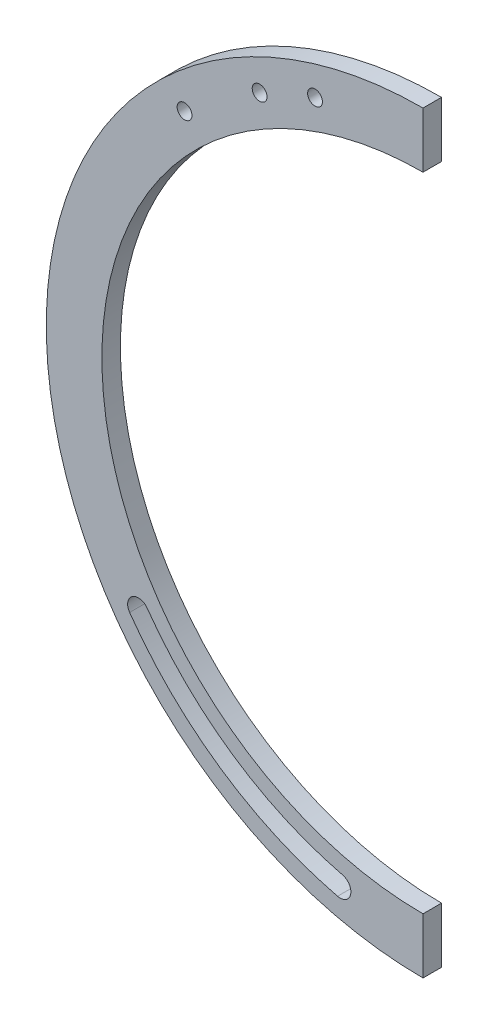
SolidWorks part; units mm, degrees
ref_plane "Front Plane" through (0, 0, 0) normal (0, 0, 1) x (1, 0, 0)
ref_plane "Top Plane" through (0, 0, 0) normal (0, 1, 0) x (1, 0, 0)
ref_plane "Right Plane" through (0, 0, 0) normal (1, 0, 0) x (0, 0, -1)
sketch "Sketch1" plane through (0, 0, 0) normal (0, 0, 1) x (1, 0, 0)
  circle A0 centre (291.5852, 182.7307) radius 203.2949
  circle A1 centre (291.5852, 182.7307) radius 173.2949
  arc A2 (93.8621, 230) -> (110.6713, 90) centre (291.5852, 182.7307) ccw construction
  dimension "D1" = 30
extrude "Boss-Extrude1" add sketch "Sketch1" against normal blind 10
sketch "Sketch2" plane through (0, 0, -10) normal (0, 0, -1) x (-1, 0, 0)
  line L0 (-291.5852, 9.4358) -> (-291.5852, -33.9055)
  line L1 (-291.5852, 356.0256) -> (-291.5852, 399.3669)
  circle A0 centre (-291.5852, 182.7307) radius 173.2949 construction
  arc A1 (-291.5852, 356.0256) -> (-291.5852, 9.4358) centre (-291.5852, 182.7307) ccw
  arc A2 (-291.5852, 399.3669) -> (-291.5852, -33.9055) centre (-291.5852, 182.7307) ccw
extrude "Cut-Extrude1" cut sketch "Sketch2" against normal blind 185
sketch "Sketch3" plane through (0, 0, -10) normal (0, 0, -1) x (-1, 0, 0)
  arc A0 (-246.849, 0.2333) -> (-138.0051, 74.4728) centre (-291.5852, 182.7307) ccw construction
  arc A1 (-245.4633, -5.4196) -> (-133.2479, 71.1194) centre (-291.5852, 182.7307) ccw
  arc A2 (-248.2347, 5.8862) -> (-142.7622, 77.8261) centre (-291.5852, 182.7307) ccw
  arc A3 (-248.2347, 5.8862) -> (-245.4633, -5.4196) centre (-246.849, 0.2333) ccw
  arc A4 (-133.2479, 71.1194) -> (-142.7622, 77.8261) centre (-138.0051, 74.4728) ccw
  point P5 (-185.7069, 27.5005)
extrude "Cut-Extrude2" cut sketch "Sketch3" against normal blind 185
sketch "Sketch4" plane through (0, 0, -10) normal (0, 0, -1) x (-1, 0, 0)
  circle A0 centre (-203.4116, 349.105) radius 4
  circle A1 centre (-233.3177, 361.7834) radius 4
  circle A3 centre (-162.898, 320.1883) radius 4
extrude "Cut-Extrude3" cut sketch "Sketch4" against normal through all both and the other way through all
